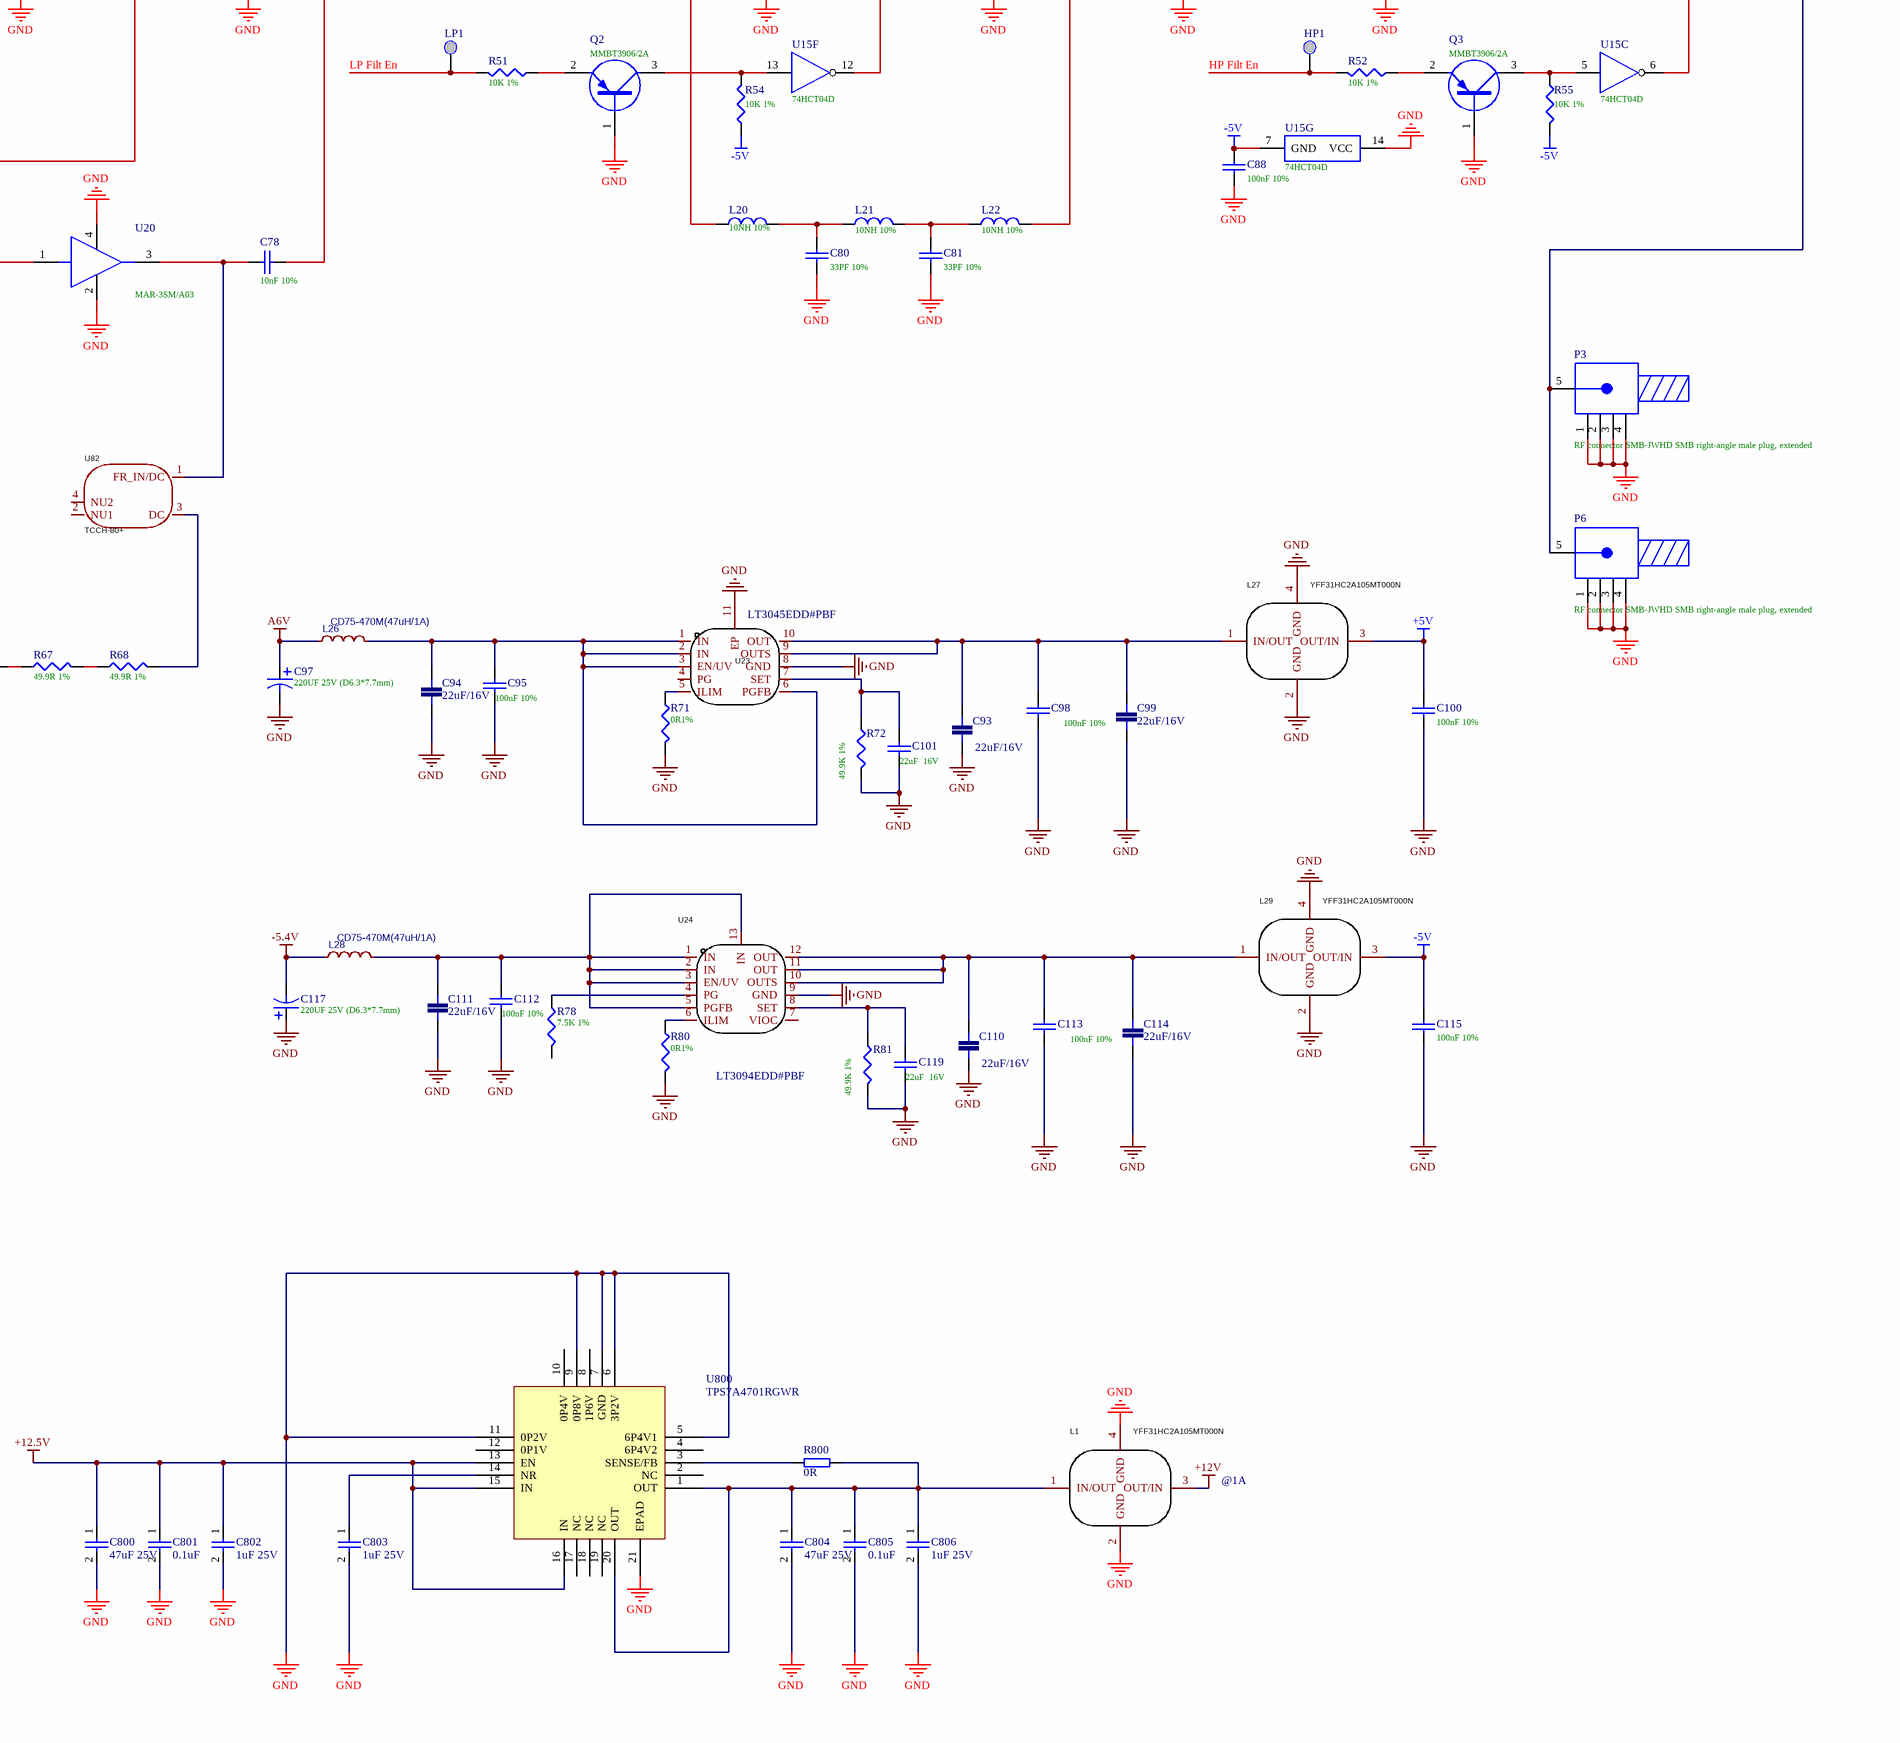
[diagram p0: PCBE109560-3.SchDoc, bottom right]
# Altium schematic sheet PCBE109560-3.SchDoc (part 2 of 2)

## Parts
1  (no value)  [DIP-1]
+1  (no value)  [DIP-1]
+2  (no value)  [DIP-1]
C4  20PF 10%  [0805C-2]
C5  330PF 10%  [1812C]
C6  22PF 10%  [1812C-2]
C7  22uF/16V  [0805]
C8  22uF/16V  [0805]
C9  100nF 10%  [0603]
C10  220UF 25V (D6.3*7.7mm)  [CAP-SMD_BD6.3-L6.6-W6.6-FD]
C11  100nF 10%  [0603]
C12  22uF/16V  [0805]
C13  100nF 10%  [0805R]
C14  22uF  16V  [0805]
C15  100nF 10%  [0805R]
C16  47PF 10%  [1812C-2]
C17  100PF 10%  [1812C-2]
C18  20PF 10%  [0805R]
C20  100nF 10%  [0805R]
C21  100nF 10%  [0805R]
C31  100nF 10%  [0805R]
C32  100nF 10%  [0805R]
C34  100nF 10%  [0805R]
C35  100nF 10%  [0805R]
C36  100nF 10%  [0805R]
C37  100nF 10%  [0805R]
C39  100nF 10%  [0805R]
C40  100nF 10%  [0805R]
C41  100nF 10%  [0805R]
C42  100nF 10%  [0805R]
C43  100nF 10%  [0805R]
C44  100nF 10%  [0805R]
C45  100nF 10%  [0805R]
C46  100nF 10%  [0805R]
C47  100nF 10%  [0805R]
C48  100nF 10%  [0805R]
C49  22uF 25V  [CAP-SMD_L6.0-W3.2-R-RD]
C50  100nF 10%  [0805R]
C51  100nF 10%  [0805R]
C52  100nF 10%  [0805R]
C53  3.3NF 10%  [0805R]
C54  100nF 10%  [0805R]
C55  330PF 10%  [0805R]
C56  330PF 10%  [0805R]
C57  100nF 10%  [0805R]
C58  33PF 10%  [0805R]
C59  33PF 10%  [0805R]
C60  100nF 10%  [0805R]
C61  100nF 10%  [0805R]
C62  100nF 10%  [0805R]
C63  100nF 10%  [0805R]
C64  100nF 10%  [0805R]
C65  33PF 10%  [0805R]
C66  33PF 10%  [0805R]
C67  100nF 10%  [0805R]
C68  39PF 10%  [0805R]
C69  100nF 10%  [0805R]
C70  25V 1UF Type A  [0805C-2]
C71  25V 1UF Type A  [0805C-2]
C72  100nF 10%  [0805R]
C73  25V 1UF Type A  [0805C-2]
C74  100nF 10%  [0805R]
C75  100nF 10%  [0805R]
C76  10nF 10%  [0805R]
C77  10nF 10%  [0805R]
C78  10nF 10%  [0805R]
C79  100nF 10%  [0603C]
C80  33PF 10%  [0805R]
C81  33PF 10%  [0805R]
C82  100nF 10%  [0805R]
C83  100nF 10%  [0805R]
C84  100nF 10%  [0805R]
C85  100nF 10%  [0805R]
C86  25V 1UF Type A  [0805C-2]
C87  3pF( ±0.1pF)  [0805R]
C88  100nF 10%  [0805R]
C89  100nF 10%  [0805R]
C90  100nF 10%  [0805R]
C93  22uF/16V  [0805]
C94  22uF/16V  [0805]
C95  100nF 10%  [0603]
C96  100nF 10%  [0805R]
C97  220UF 25V (D6.3*7.7mm)  [CAP-SMD_BD6.3-L6.6-W6.6-FD]
C98  100nF 10%  [0603]
C99  22uF/16V  [0805]
C100  100nF 10%  [0805R]
C101  22uF  16V  [0805]
C102  100nF 10%  [0805R]
C103  100nF 10%  [0805R]
C104  100nF 10%  [0805R]
C105  100nF 10%  [0805R]
C106  100nF 10%  [0805R]
C107  100nF 10%  [0805R]
C109  100nF 10%  [0805R]
C110  22uF/16V  [0805]
C111  22uF/16V  [0805]
C112  100nF 10%  [0603]
C113  100nF 10%  [0603]
C114  22uF/16V  [0805]
C115  100nF 10%  [0805R]
C116  100nF 10%  [0805R]
C117  220UF 25V (D6.3*7.7mm)  [CAP-SMD_BD6.3-L6.6-W6.6-FD]
C118  100nF 10%  [0805R]
C119  22uF  16V  [0805]
C122  100nF 10%  [0805R]
C123  100nF 10%  [0805R]
C124  100nF 10%  [0805R]
C125  100nF 10%  [0805R]
C128  100nF 10%  [0805R]
C129  100nF 10%  [0805R]
C130  100nF 10%  [0805R]
C800  47uF 25V  [1206]
C801  0.1uF  [0402]
C802  1uF 25V  [0402]
C803  1uF 25V  [0402]
C804  47uF 25V  [1206]
C805  0.1uF  [0402]
C806  1uF 25V  [0402]
C809  100nF 10%  [0805R]
C888  100nF 10%  [0805R]
Clk1  (no value)  [DIP-1]
D1  BAV99/A7  [SOT-23]
D2  GF1M-E3/67A/GM  [1808D]
D3  GF1M-E3/67A/GM  [1808D]
D4  GF1M-E3/67A/GM  [1808D]
D5  GF1M-E3/67A/GM  [1808D]
D8  BAV99/A7  [SOT-23-2]
D9  BAV99/A7  [SOT-23-2]
D10  BAV99/A7  [SOT-23-2]
D11  BAV99/A7  [SOT-23-2]
D12  BAV99/A7  [SOT-23-2]
Data1  (no value)  [DIP-1]
HP1  (no value)  [DIP-1]
J1  RF connector  [DIP-P]
J2  RF connector  [DIP-P]
L1  YFF31HC2A105MT000N  [FILTER-SMD_4P-L3.2-W1.6-L_YFF31HC]
L2  15UH 5%  [1005R]
L3  BLM21PG221SN1D(220Ω@100MHz)  [0805R]
L4  YFF31HC2A105MT000N  [FILTER-SMD_4P-L3.2-W1.6-L_YFF31HC]
L5  6.8UH 10%  [0805R]
L8  YFF31HC2A105MT000N  [FILTER-SMD_4P-L3.2-W1.6-L_YFF31HC]
L10  10NH 10%  [0805R]
L11  10NH 10%  [0805R]
L12  10NH 10%  [0805R]
L13  YFF31HC2A105MT000N  [FILTER-SMD_4P-L3.2-W1.6-L_YFF31HC]
L15  4.7UH 5%  [1005L]
L16  1UH 5%  [0805R]
L17  BLM21PG221SN1D(220Ω@100MHz)  [0805R]
L18  BLM21PG221SN1D(220Ω@100MHz  [0805R]
L19  NFM15PC104R1A3D  [FILTER-SMD_0402-3P-L1.0-W0.5-T]
L20  10NH 10%  [0805R]
L21  10NH 10%  [0805R]
L22  10NH 10%  [0805R]
L23  YFF31HC2A105MT000N  [FILTER-SMD_4P-L3.2-W1.6-L_YFF31HC]
L24  YFF31HC2A105MT000N  [FILTER-SMD_4P-L3.2-W1.6-L_YFF31HC]
L25  BLM21PG221SN1D(220Ω@100MHz  [0805R]
L26  CD75-470M(47uH/1A)  [IND-SMD_L7.8-W7.0-A]
L27  YFF31HC2A105MT000N  [FILTER-SMD_4P-L3.2-W1.6-L_YFF31HC]
L28  CD75-470M(47uH/1A)  [IND-SMD_L7.8-W7.0-A]
L29  YFF31HC2A105MT000N  [FILTER-SMD_4P-L3.2-W1.6-L_YFF31HC]
L31  BLM21PG221SN1D(220Ω@100MHz  [0805R]
L32  BLM21PG221SN1D(220Ω@100MHz  [0805R]
L808  NFM15PC104R1A3D  [FILTER-SMD_0402-3P-L1.0-W0.5-T]
L809  NFM15PC104R1A3D  [FILTER-SMD_0402-3P-L1.0-W0.5-T]
L810  NFM15PC104R1A3D  [FILTER-SMD_0402-3P-L1.0-W0.5-T]
L811  NFM15PC104R1A3D  [FILTER-SMD_0402-3P-L1.0-W0.5-T]
L812  NFM15PC104R1A3D  [FILTER-SMD_0402-3P-L1.0-W0.5-T]
L813  NFM15PC104R1A3D  [FILTER-SMD_0402-3P-L1.0-W0.5-T]
LP1  (no value)  [DIP-1]
P1  Header 20X2  [N0.8mm/40Pin-Plug]
P2  Header 4X2  [N0.8mm/8Pin-SOCKET]
P3  RF connector SMB-JWHD SMB right-angle male plug, extended  [DIP-P-2]
P4  Header 20X2  [N0.8mm/40Pin-Plug]
P5  Header 20X2  [N0.8mm/40Pin-Plug]
P6  RF connector SMB-JWHD SMB right-angle male plug, extended  [DIP-P-2]
Q1  MJD31C  [SOT-252-2]
Q2  MMBT3906/2A  [SOT-23]
Q3  MMBT3906/2A  [SOT-23]
Q4  MMBT3906/2A  [SOT-23]
R6  2K 5%  [0603]
R7  NC  [AXIAL-0.51]
R8  3.9K 5% 1/2W  [AXIAL-0.51]
R9  3.9K 5% 1/2W  [AXIAL-0.51]
R10  3.9K 5% 1/2W  [AXIAL-0.51]
R11  3.9K 5% 1/2W  [AXIAL-0.51]
R13  0R1%  [0603]
R14  49.9K 1%  [0603]
R15  4.99K 1%  [0805R]
R16  2K 1%  [0805R]
R17  49.9R 1% 1/4W  [AXIAL-0.4]
R20  100R 1% 1/4W  [AXIAL-0.4]
R23  100R 1% 1/4W  [AXIAL-0.4]
R27  4.87K 1%  [0805R]
R28  4.87K 1%  [0805R]
R29  4.87K 1%  [0805R]
R30  4.87K 1%  [0805R]
R31  4.87K 1%  [0805R]
R32  10K 1%  [0805R]
R33  100K 1%  [0805R]
R34  100K 1%  [0805R]
R35  49.9R 1%  [0805R]
R36  49.9R 1%  [0805R]
R37  49.9R 1%  [0805R]
R38  49.9R 1%  [0805R]
R39  49.9R 1%  [0805R]
R40  49.9R 1% 1/4W  [R-SMD_L3.5-W1.5]
R41  10K 1%  [0805R]
R42  4.87K 1%  [0805R]
R43  4.87K 1%  [0805R]
R44  4.87K 1%  [0805R]
R45  4.87K 1%  [0805R]
R46  169R 1%  [0805R]
R47  169R 1%  [0805R]
R48  169R 1%  [0805R]
R49  49.9R 1%  [0805R]
R50  49.9R 1%  [0805R]
R51  10K 1%  [0805R]
R52  10K 1%  [0805R]
R53  10K 1%  [0805R]
R54  10K 1%  [0805R]
R55  10K 1%  [0805R]
R56  10K 1%  [0805R]
R57  10K 1%  [0805R]
R58  49.9R 1%  [0805R]
R59  4.99K 1%  [0805R]
R60  49.9R 1%  [R-SMD_L3.5-W1.5]
R61  30R 1%  [R-SMD_L3.5-W1.5]
R62  169R 1%  [0805R]
R63  169R 1%  [0805R]
R64  169R 1%  [0805R]
R65  49.9R 1%  [0805R]
R66  49.9R 1%  [0805R]
R67  49.9R 1%  [0805R]
R68  49.9R 1%  [0805R]
R69  120R 1%  [R-SMD_L3.5-W1.5]
R70  169R 1%  [0805R]
R71  0R1%  [0603]
R72  49.9K 1%  [0603]
R73  169R 1%  [0805R]
R74  NC  [0805R]
R75  169R 1%  [0805R]
R77  169R 1%  [0805R]
R78  7.5K 1%  [0603]
R80  0R1%  [0603]
R81  49.9K 1%  [0603]
R82  100K 1%  [0805R]
R83  10K 1%  [0805R]
R84  169R 1%  [0805R]
R800  0R  [0402]
RE1  AGQ210A4HZ  [RELAY-SMD_PANASONIC_AGQ2X0AXX]
RE2  AGQ210A4HZ  [RELAY-SMD_PANASONIC_AGQ2X0AXX]
RE3  AGQ210A4HZ  [RELAY-SMD_PANASONIC_AGQ2X0AXX]
RE4  AGQ210A4HZ  [RELAY-SMD_PANASONIC_AGQ2X0AXX]
RE5  AGQ210A4HZ  [RELAY-SMD_PANASONIC_AGQ2X0AXX]
Strobe1  (no value)  [DIP-1]
U4  LT3045EDD#PBF  [DFN-10_L3.0-W3.0-P0.50-BL-EP]
U6  74HCT123D  [SOIC-16_L9.9-W3.9-P1.27-LS6.0-BL]
U8  MAX504CSD+T  [SO-14]
U9  SW-239  [SO-8]
U11  SW-239  [SO-8]
U12  SW-239  [SO-8]
U13  SW-239  [SO-8]
U14  SW-239  [SO-8]
U15  74HCT04D  [SO-14]  (parts A,B,C,D,E,F,G of 7)
U16  AT-250(MAAV-007941)  [SO-8]
U17  MAR-3SM/A03  [LCC4]
U18  MAR-6SM/A06  [LCC4]
U19  MAR-6SM/A06  [LCC4]
U20  MAR-3SM/A03  [LCC4]
U21  MAX4106ESA+T  [SO-8]
U22  MIC4420CM  [SO-8]
U23  LT3045EDD#PBF  [DFN-10_L3.0-W3.0-P0.50-BL-EP]
U24  LT3094EDD#PBF  [WDFN-12_L3.0-W3.0-P0.45-BL-EP]
U25  AT65-0263  [SO-16]
U80  TCCH-80+  [IND-SMD_4P-L3.8-W3.8]
U81  TCCH-80+  [IND-SMD_4P-L3.8-W3.8]
U82  TCCH-80+  [IND-SMD_4P-L3.8-W3.8]
U83  TCCH-80+  [IND-SMD_4P-L3.8-W3.8]
U100  SW-239  [SO-8]
U800  TPS7A4701RGWR  [QFN-20]

## Nets
+5V: C100.1 C888.1 L25.1 L27.3(OUT/IN) L811.3(OUTPUT) L812.3(OUTPUT) U8.3(~{CLR})
+12.5V: +2.1 C106.1 C800.1 C801.1 C802.1 P5.31 P5.32 P5.33 P5.34 P5.35 P5.36 P5.37 P5.38 P5.39 P5.40 U800.13(EN) U800.15(IN) U800.16(IN)
+12V: C122.1 C123.1 C124.2 C125.2 L1.3(OUT/IN) L8.1(IN/OUT) L13.1(IN/OUT) U22.1(VS) U22.8(VS)
-5.4V: +1.1 C107.1 C117.2 L28.2 P5.1 P5.2 P5.3 P5.4 P5.5 P5.6 P5.7 P5.8 P5.9 P5.10
-5V: C88.2 C115.2 L29.3(OUT/IN) L809.1(INPUT) L810.3(OUTPUT) L813.3(OUTPUT) R54.1 R55.2 R57.1 U15.7(GND)
A6V: 1.1 C10.1 C97.1 C103.2 L3.1 L26.2 P5.17 P5.18 P5.19 P5.20 P5.21 P5.22 P5.23 P5.24
GND: C5.1 C6.2 C7.1 C8.1 C9.2 C10.2 C11.2 C12.1 C13.2 C14.2 C15.1 C18.2 C20.1 C21.1 C31.1 C32.1 C34.1 C35.1 C36.2 C37.2 C39.2 C40.2 C42.2 C43.1 C44.2 C45.2 C46.2 C47.1 C48.1 C49.2 C50.2 C57.2 C60.2 C61.1 C62.1 C63.1 C64.1 C65.2 C66.1 C70.1 C71.1 C72.2 C73.1 C74.1 C75.1 C80.1 C81.1 C83.2 C84.2 C85.1 C86.2 C88.1 C89.2 C90.2 C93.1 C94.1 C95.2 C96.2 C97.2 C98.2 C99.1 C100.2 C101.2 C102.2 C103.1 C104.2 C105.1 C106.2 C107.2 C109.2 C110.1 C111.1 C112.2 C113.2 C114.1 C115.1 C117.1 C118.2 C119.2 C122.2 C123.2 C124.1 C125.1 C128.1 C129.1 C130.2 C800.2 C801.2 C802.2 C803.2 C804.2 C805.2 C806.2 C809.2 C888.2 D1.3 D2.2(K) D11.2 D12.1 J1.1 J1.2 J1.3 J1.4 J2.1 J2.2 J2.3 J2.4 L1.2(GND) L1.4(GND) L2.2 L4.2(GND) L4.4(GND) L8.2(GND) L8.4(GND) L13.2(GND) L13.4(GND) L15.2 L16.1 L19.2(GND) L23.2(GND) L23.4(GND) L24.2(GND) L24.4(GND) L27.2(GND) L27.4(GND) L29.2(GND) L29.4(GND) L808.2(GND) L809.2(GND) L810.2(GND) L811.2(GND) L812.2(GND) L813.2(GND) P1.5 P1.6 P1.11 P1.12 P1.17 P1.18 P1.20 P1.23 P1.24 P1.29 P1.30 P1.35 P1.36 P2.1 P2.3 P2.5 P2.7 P3.1 P3.2 P3.3 P3.4 P4.5 P4.6 P4.11 P4.12 P4.17 P4.18 P4.23 P4.24 P4.29 P4.30 P4.35 P4.36 P5.11 P5.12 P5.13 P5.14 P5.15 P5.16 P5.25 P5.26 P5.27 P5.28 P5.29 P5.30 P6.1 P6.2 P6.3 P6.4 Q1.2(E) Q2.1(B) Q3.1(B) Q4.1(B) R13.2 R14.2 R20.2 R32.2 R53.1 R59.1 R61.1 R71.2 R72.2 R74.1 R80.2 R81.2 R82.1 R83.1 RE1.3 RE3.6 RE4.2 U4.8(GND) U4.11(EP) U6.6(2CEXT) U6.8(GND) U6.10(2B) U6.14(1CEXT) U8.7(DGND) U8.8(AGND) U9.2(GND) U9.7(GND) U9.8(GND) U11.2(GND) U11.7(GND) U11.8(GND) U12.2(GND) U12.7(GND) U12.8(GND) U13.2(GND) U13.7(GND) U13.8(GND) U14.2(GND) U14.7(GND) U14.8(GND) U15.14(VCC) U16.2(GND) U16.3(GND) U16.5(GND) U16.6(GND) U16.7(GND) U17.2(GND) U17.4(GND) U18.2(GND) U18.4(GND) U19.2(GND) U19.4(GND) U20.2(GND) U20.4(GND) U22.4(GND) U22.5(GND) U23.8(GND) U23.11(EP) U24.9(GND) U25.2(GND) U25.3(GND) U25.4(GND) U25.5(GND) U25.6(GND) U25.7(GND) U25.16(GND) U100.2(GND) U100.7(GND) U100.8(GND) U800.5(6P4V1) U800.6(3P2V) U800.7(GND) U800.9(0P8V) U800.11(0P2V) U800.21(EPAD)
VCC: C13.1 C15.2 L4.3(OUT/IN) R15.1 R16.2 U6.2(1B) U6.3(1~{R}D) U6.16(VCC)
AK2: C21.2 P1.33 RE1.1
AK3: C20.2 P1.38 RE1.8
AK4: C37.1 P1.37 RE2.1
AK5: C36.1 P1.40 RE2.8
AK6: C31.2 P1.34 RE3.8
AK7: C32.2 P1.32 RE3.1
AK8: C34.2 C40.1 P1.28 RE4.8 RE5.8
AK9: C35.2 C39.1 P1.26 RE4.1 RE5.1
Attn1: P4.34 R70.2
Attn2: P4.32 R73.2
Attn4: P4.28 R75.2
Attn8: P4.26 R77.2
Attn16: P4.22 R84.2
DAC Clk: Clk1.1 P4.14 U8.4(SCLK)
DAC Data: Data1.1 P4.16 U8.2(DIN)
DAC Strobe: P4.10 Strobe1.1 U8.5(~{CS})
DATA_T: P1.39 R15.2 U6.1(1~{A})
HP Filt En: HP1.1 P4.4 R52.2
HT: L5.1 P2.2 P2.4 P2.6 P2.8
IN2: P4.8 R56.1 U22.2(IN)
LP Filt En: LP1.1 P4.2 R51.2
NetC4_1: C4.1 D1.2 L2.1 Q1.1(B) R6.1
NetC4_2: C4.2 R6.2 U6.13(1Q)
NetC5_2: C5.2 L5.2 R7.2
NetC6_1: C6.1 C16.2 C17.2 Q1.3(C) R11.1
NetC7_2: C7.2 C11.1 C12.2 L4.1(IN/OUT) U4.9(OUTS) U4.10(OUT)
NetC8_2: C8.2 C9.1 L3.2 U4.1(IN) U4.2(IN) U4.3(EN/UV) U4.6(PGFB)
NetC14_1: C14.1 R14.1 U4.7(SET)
NetC16_1: C16.1 D5.1(A) D8.2 D9.2 RE2.6
NetC17_1: C17.1 RE2.7
NetC18_1: C18.1 R16.1 U6.15(1REXT/CEXT)
NetC41_1: C41.1 U14.1(RFCOM)
NetC41_2: C41.2 P3.5 P6.5 R32.1
NetC42_1: C42.1 R27.1 U9.5(B)
NetC43_2: C43.2 R28.2 U100.4(A)
NetC44_1: C44.1 R29.1 U11.4(A)
NetC45_1: C45.1 R30.1 U12.5(B)
NetC46_1: C46.1 R31.1 U13.5(B) U14.4(A)
NetC47_2: C47.2 R35.1 U16.4(A)
NetC48_2: C48.2 L8.3(OUT/IN) R36.1
NetC49_1: C49.1 C50.1 U8.1(BIPOFF) U8.9(REFIN) U8.10(REFOUT)
NetC51_1: C51.1 U17.1(RF_IN)
NetC51_2: C51.2 U16.8(RF2)
NetC52_1: C52.1 L10.2
NetC52_2: C52.2 U17.3(RF_OUT) U81.1(FR_IN/DC)
NetC53_1: C53.1 C54.1 L15.1
NetC53_2: C53.2 U12.1(RFCOM)
NetC54_2: C54.2 U13.1(RFCOM)
NetC55_1: C55.1 U13.3(RF1)
NetC55_2: C55.2 C56.1 L16.2
NetC56_2: C56.2 U14.6(RF2)
NetC57_1: C57.1 R41.1 U13.4(A) U14.5(B)
NetC58_1: C58.1 C65.1
NetC58_2: C58.2 L10.1 L11.1
NetC59_1: C59.1 L11.2 L12.1
NetC59_2: C59.2 C66.2
NetC60_1: C60.1 R42.1 U9.4(A)
NetC61_2: C61.2 R43.2 U100.5(B)
NetC62_2: C62.2 R44.1 U11.5(B)
NetC63_2: C63.2 R45.1 U12.4(A)
NetC64_2: C64.2 L13.3(OUT/IN) R46.2
NetC67_1: C67.1 U18.1(RF_IN)
NetC67_2: C67.2 U25.1(RF)
NetC68_1: C68.1 C69.2 R49.2 R50.2
NetC68_2: C68.2 R49.1 R50.1 U18.3(RF_OUT) U80.1(FR_IN/DC)
NetC69_1: C69.1 R53.2 U16.1(RF1)
NetC70_2: C70.2 C74.2 L18.1 L19.1(INPUT)
NetC71_2: C71.2 C75.2 L19.3(OUTPUT) U21.4(VEE)
NetC72_1: C72.1 C73.2 L17.2 L18.2
NetC76_1: C76.1 U9.3(RF1)
NetC76_2: C76.2 U19.1(RF_IN)
NetC77_1: C77.1 U19.3(RF_OUT) U83.1(FR_IN/DC)
NetC77_2: C77.2 U20.1(RF_IN)
NetC78_1: C78.1 U20.3(RF_OUT) U82.1(FR_IN/DC)
NetC78_2: C78.2 U100.6(RF2)
NetC79_1: C79.1 D10.3 R40.2
NetC79_2: C79.2 R58.2 R59.2
NetC80_2: C80.2 L20.2 L21.2
NetC81_2: C81.2 L21.1 L22.1
NetC82_1: C82.1 R60.2
NetC82_2: C82.2 C116.1 R74.2 R82.2
NetC83_1: C83.1 C86.1 L808.1(INPUT) U21.7(VCC)
NetC84_1: C84.1 L23.3(OUT/IN) R62.2
NetC85_2: C85.2 L24.3(OUT/IN) R65.1
NetC87_1: C87.1 R60.1 R69.1 U21.6(OUT)
NetC87_2: C87.2 R61.2 R69.2 U21.2(IN-)
NetC89_1: C89.1 L813.1(INPUT) U8.11(VSS)
NetC90_1: C90.1 L32.2 L811.1(INPUT)
NetC93_2: C93.2 C98.1 C99.2 L27.1(IN/OUT) U23.9(OUTS) U23.10(OUT)
NetC94_2: C94.2 C95.1 L26.1 U23.1(IN) U23.2(IN) U23.3(EN/UV) U23.6(PGFB)
NetC96_1: C96.1 R70.1 U25.15(C1)
NetC101_1: C101.1 R72.1 U23.7(SET)
NetC102_1: C102.1 R73.1 U25.14(C2)
NetC104_1: C104.1 L812.1(INPUT) U8.13(VDD)
NetC105_2: C105.2 L31.1 L810.1(INPUT)
NetC109_1: C109.1 R75.1 U25.13(C4)
NetC110_2: C110.2 C113.1 C114.2 L29.1(IN/OUT) U24.10(OUTS) U24.11(OUT) U24.12(OUT)
NetC111_2: C111.2 C112.1 L28.1 U24.1(IN) U24.2(IN) U24.3(EN/UV) U24.5(PGFB) U24.13(IN)
NetC116_2: C116.2 R83.2 U25.8(RF)
NetC118_1: C118.1 R77.1 U25.12(C8)
NetC119_1: C119.1 R81.1 U24.8(SET)
NetC128_2: C128.2 L31.2 U25.11(VEE)
NetC129_2: C129.2 L32.1 U25.10(VCC)
NetC130_1: C130.1 R84.1 U25.9(C16)
NetC803_1: C803.1 U800.14(NR)
NetC804_1: C804.1 C805.1 C806.1 L1.1(IN/OUT) R800.1 U800.1(OUT) U800.20(OUT)
NetC809_1: C809.1 L25.2 L808.3(OUTPUT)
NetD2_1: D2.1(A) D3.2(K)
NetD3_1: D3.1(A) D4.2(K)
NetD4_1: D4.1(A) D5.2(K)
NetD8_1: D8.1 D9.1 J1.5 R17.1 R20.1 R23.1 RE4.4
NetD10_1: D10.1 D12.2
NetD10_2: D10.2 D11.1
NetJ2_5: J2.5 RE5.4
NetL12_2: L12.2 U9.1(RFCOM)
NetL17_1: L17.1 L809.3(OUTPUT)
NetL20_1: L20.1 U11.6(RF2)
NetL22_2: L22.2 U12.3(RF1)
NetL23_1: L23.1(IN/OUT) L24.1(IN/OUT) U22.6(OUT) U22.7(OUT)
NetQ2_2: Q2.2(E) R51.1
NetQ2_3: Q2.3(C) R54.2 U15.13(6A)
NetQ3_2: Q3.2(E) R52.1
NetQ3_3: Q3.3(C) R55.1 U15.5(3A)
NetQ4_2: Q4.2(E) R56.2
NetQ4_3: Q4.3(C) R57.2 U15.1(1A)
NetR7_1: R7.1 R8.1
NetR8_2: R8.2 R9.2
NetR9_1: R9.1 R10.1
NetR10_2: R10.2 R11.2
NetR13_1: R13.1 U4.5(ILIM)
NetR17_2: R17.2 RE1.2
NetR23_2: R23.2 RE3.7
NetR27_2: R27.2 R28.1 U15.4(2Y)
NetR29_2: R29.2 R30.2 U15.10(5Y)
NetR31_2: R31.2 U15.8(4Y)
NetR33_1: R33.1 R34.1 U8.14(RFB)
NetR33_2: R33.2 R34.2 R35.2 U8.12(VOUT)
NetR36_2: R36.2 R37.1
NetR37_2: R37.2 R38.2
NetR38_1: R38.1 R39.1
NetR39_2: R39.2 U81.3(DC)
NetR40_1: R40.1 RE5.3
NetR41_2: R41.2 U15.6(3Y) U15.9(4A)
NetR42_2: R42.2 R43.1 U15.2(1Y) U15.3(2A)
NetR44_2: R44.2 R45.2 U15.11(5A) U15.12(6Y)
NetR46_1: R46.1 R47.2
NetR47_1: R47.1 R48.1
NetR48_2: R48.2 U80.3(DC)
NetR58_1: R58.1 U21.3(IN+)
NetR62_1: R62.1 R63.1
NetR63_2: R63.2 R64.2
NetR64_1: R64.1 U83.3(DC)
NetR65_2: R65.2 R66.2
NetR66_1: R66.1 R67.1
NetR67_2: R67.2 R68.1
NetR68_2: R68.2 U82.3(DC)
NetR71_1: R71.1 U23.5(ILIM)
NetR78_1: R78.1 U24.4(PG)
NetR80_1: R80.1 U24.6(ILIM)
NetR800_2: R800.2 U800.3(SENSE/FB)
NetRE4_3: RE4.3 RE5.2
NetU9_6: U9.6(RF2) U100.3(RF1)
NetU11_1: U11.1(RFCOM) U100.1(RFCOM)
NetU11_3: U11.3(RF1) U12.6(RF2)
NetU13_6: U13.6(RF2) U14.3(RF1)

Not connected (* = marked no-connect by the designer): D1 1*; D8 3; D9 3; D11 3; D12 3; P1 1 2 3 4 7 8 9 10 13 14 15 16 19 21 22 25 27 31; P4 1 3 7 9 13 15 19 20 21 25 27 31 33 37 38 39 40; R78 2; RE1 4 5 6 7; RE2 2 3 4 5; RE3 2 3 4 5; RE4 5 6 7; RE5 5 6 7; U4 4(PG); U6 4(1~{Q}) 5(2Q) 7(2REXT/CEXT) 9(2~{A}) 11(2~{R}D) 12(2~{Q}); U8 6(DOUT); U22 3(NC); U23 4(PG); U24 7(VIOC); U80 2(NU1) 4(NU2); U81 2(NU1) 4(NU2); U82 2(NU1) 4(NU2); U83 2(NU1) 4(NU2); U800 2(NC) 4(6P4V2) 8(1P6V) 10(0P4V) 12(0P1V) 17(NC) 18(NC) 19(NC)

## Notes on the sheet
- (near P1) Transmit interface
- 500V high-voltage interface
- Receive interface
- @1A

## Library data of the parts
1 +1 +2 Clk1 Data1 HP1 LP1 Strobe1 = TP
C4-C6 C9 C11 C13-C18 C20 C21 C31 C32 C34-C37 C39-C48 C50-C69 C72-C85 C87-C90 C95 C96 C98 C100-C107 C109 C112 C113 C115 C116 C118 C119 C122-C125 C128-C130 C800-C806 C809 C888 = CAP: Capacitor
C7 C8 C12 C93 C94 C99 C110 C111 C114 = C1206
C10 C97 C117 = CAPACITOR_1: Capacitor
C49 = TAJC226K025RNJ: Manufacturer: Kyocera AVX; Add into BOM: yes; Tolerance: ±10%; Equivalent Series Resistance(ESR): 1.4Ω@100kHz; Symbol: TAJC226K025RNJ; Device: TAJC226K025RNJ; LCSC Part Name: 22uF ±10% 25V; Supplier Part: C7214; Manufacturer Part: TAJC226K025RNJ; Supplier Footprint: CASE-C-6032; JLCPCB Part Class: Extended Part; Datasheet: https://atta.szlcsc.com/upload/public/pdf/source/20160107/1457707750344.pdf; Supplier: LCSC; Convert to PCB: yes; Value: 22uF; Rated Voltage: 25V; Operating Temperature: -55℃~+125℃
C70 C71 C86 = CAPACITOR POL: Capacitor
D1 D8-D12 = BAV99
D2-D5 = DIODE
J1 J2 = SMA-KWE: BOM_Supplier: *; BOM_Supplier Part: *; BOM_Manufacturer: *; BOM_Manufacturer Part: *; BOM_JLCPCB Part Class: *; spicePre: *; spiceSymbolName: *; Contributor: *
L1 L4 L8 L13 L23 L24 L27 L29 = YFF31HC2A105MT000N: Manufacturer: TDK; Add into BOM: yes; Nominal Capacitance: 1uF; CapacitanceTolerance: ±20%; DC Rated Voltage: 100V; Rated Current: 6A; DC Resistance: 5mΩ; Name: YFF31HC2A105MT000N; Symbol: YFF31HC2A105MT000N; Device: YFF31HC2A105MT000N; LCSC Part Name: 1uF(105) ±20% 100V; Supplier Part: C113216; Manufacturer Part: YFF31HC2A105MT000N; Supplier Footprint: SMD-4P,1.6x3.2mm; JLCPCB Part Class: Extended Part; Datasheet: https://atta.szlcsc.com/upload/public/pdf/source/20180326/C113216_F6F81E50B9805DA3D7C436129903DEBD.pdf; Supplier: LCSC; Convert to PCB: yes; Operating Temperature: -55℃~+125℃
L2 L3 L5 L10-L12 L15-L18 L20-L22 L25 L31 L32 = INDUCTOR
L19 L808-L813 = NFM15PC104R1A3D: Manufacturer: muRata(村田); Add into BOM: yes; Nominal Capacitance: 100nF; CapacitanceTolerance: ±20%; DC Rated Voltage: 10V; Rated Current: 2A; DC Resistance: 30mΩ; Symbol: NFM15PC104R1A3D; Device: NFM15PC104R1A3D; LCSC Part Name: 0.1uF ±20% 10V; Supplier Part: C2650905; Manufacturer Part: NFM15PC104R1A3D; Supplier Footprint: 0402; JLCPCB Part Class: Extended Part; Datasheet: https://atta.szlcsc.com/upload/public/pdf/source/20210611/05FD8D968916F804F398094FB2B4AAFE.pdf; Supplier: LCSC; Convert to PCB: yes; Operating Temperature: -55℃~+105℃; Comment_1: NFM15PC104R1A3D
L26 L28 = 4.7uH/5a: BOM_Manufacturer: COILMX; BOM_Manufacturer Part: MS0630-4R7M; nameAlias: Inductance; Contributor: LCSC; BOM_Supplier: LCSC; BOM_Supplier Part: C380177; spicePre: L; spiceSymbolName: MS0630-4R7M
P1 P4 P5 = Header 20X2: Header, 20-Pin, Dual row; LatestRevisionDate: 17-Jul-2002; LatestRevisionNote: Re-released for DXP Platform.; Publisher: Altium Limited
P2 = Header 4X2: Header, 4-Pin, Dual row; LatestRevisionDate: 17-Jul-2002; LatestRevisionNote: Re-released for DXP Platform.; Publisher: Altium Limited
P3 P6 = JA1
Q1 = NPN: NPN Transistor
Q2-Q4 = PNP: PNP Transistor
R6-R11 R13-R17 R20 R23 R27-R75 R77 R78 R80-R84 = RES1
R800 = RES
RE1-RE5 = AGQ210A4HZ: Manufacturer: PANASONIC(松下); Add into BOM: yes; Coil Voltage: 4.5V; Contact Form: Two changeover sets: 2C (DPDT changeover); Maximum Switching Voltage: 125V@AC; 110V@DC; Coil Type: Single coil; Maximum Switching Current: 2A; Operate Time: 4ms; Symbol: AGQ210A4HZ; Device: AGQ210A4HZ; LCSC Part Name: AGQ210A4HZ; Supplier Part: C2153577; Manufacturer Part: AGQ210A4HZ; Supplier Footprint: SMD,7.2x10.6mm; JLCPCB Part Class: Extended Part; Datasheet: https://atta.szlcsc.com/upload/public/pdf/source/20210727/C2858037_82AE1FE69E1888D41D6E9B5D42950540.pdf; Supplier: LCSC; Convert to PCB: yes; Pin Number: -; Contact Rating: -; Contact Material: AgPd + gold plating; Coil Rated Power: -; Coil Resistance: -; Release Time: 4ms; Contact Resistance: -; Operating Temperature: -40℃~+85℃; Comment_1: AGQ210A4HZ
U4 U23 = LT3045EDD#PBF: Symbol: LT3045EDD#PBF_C666574; Add into BOM: yes; Maximum Input Voltage: 20V; Output Voltage: 0V~15V; MAX Output Current: 500mA; Dropout Voltage: 450mV@(500mA); standby current: 20uA; Number of Outputs: 1; Device: LT3045EDD#PBF; LCSC Part Name: LT3045EDD#PBF; Supplier Part: C666574; Manufacturer Part: LT3045EDD#PBF; Supplier Footprint: DFN-10-EP(3x3); JLCPCB Part Class: Extended Part; Datasheet: https://atta.szlcsc.com/upload/public/pdf/source/20200416/C514420_E440C492D6C74EAE6AB301243586F696.pdf; Supplier: LCSC; Convert to PCB: yes
U15 = 74HC04
U16 = AT-250
U17 U20 = MAR-3SM
U18 U19 = MAR-6SM
U21 = MAX4107ESA: Manufacturer: *; Manufacturer Part: *; Supplier Part: *; Supplier: *; link: *; spicePre: *; spiceSymbolName: *; Package Display: *; Contributor: *
U24 = LT3094EDD#PBF: Add into BOM: yes; Symbol: LT3094EDD#PBF; Device: LT3094EDD#PBF; LCSC Part Name: LT3094EDD#PBF; Supplier Part: C670492; Manufacturer Part: LT3094EDD#PBF; Supplier Footprint: WDFN-12-EP(3x3); JLCPCB Part Class: Extended Part; Datasheet: https://atta.szlcsc.com/upload/public/pdf/source/20200318/C498217_A5485280C797CF3891C55BEBE66C21D4.pdf; Supplier: LCSC; Convert to PCB: yes; Output Type: -
U80-U83 = TCCH-80+: Manufacturer: Mini-Circuits; Add into BOM: yes; Value: 4uH; Rated Current: 200mA; DC Resistance (DCR): 100mΩ; Symbol: TCCH-80+; Device: TCCH-80+; LCSC Part Name: 4uH; Supplier Part: C3223029; Manufacturer Part: TCCH-80+; Supplier Footprint: SMD-4P,3.8x3.8mm; JLCPCB Part Class: Extended Part; Datasheet: https://atta.szlcsc.com/upload/public/pdf/source/20240402/75EC49D4FFFA61CBEC009CC2CCA83C83.pdf; Supplier: LCSC; Convert to PCB: yes; Tolerance: -; Saturation Current (Isat): -; Type: -; Ratings: -
U800 = TPS7A4701RGWR(QFN20): Name: *; Symbol: *; Device: *; LCSC Part Name: *; Supplier Part: *; Manufacturer: *; Manufacturer Part: *; Supplier Footprint: *; JLCPCB Part Class: *; Datasheet: *; Supplier: *; Add into BOM: *; Convert to PCB: *; Output Type: *; Output Polarity: *; Number of Outputs: *